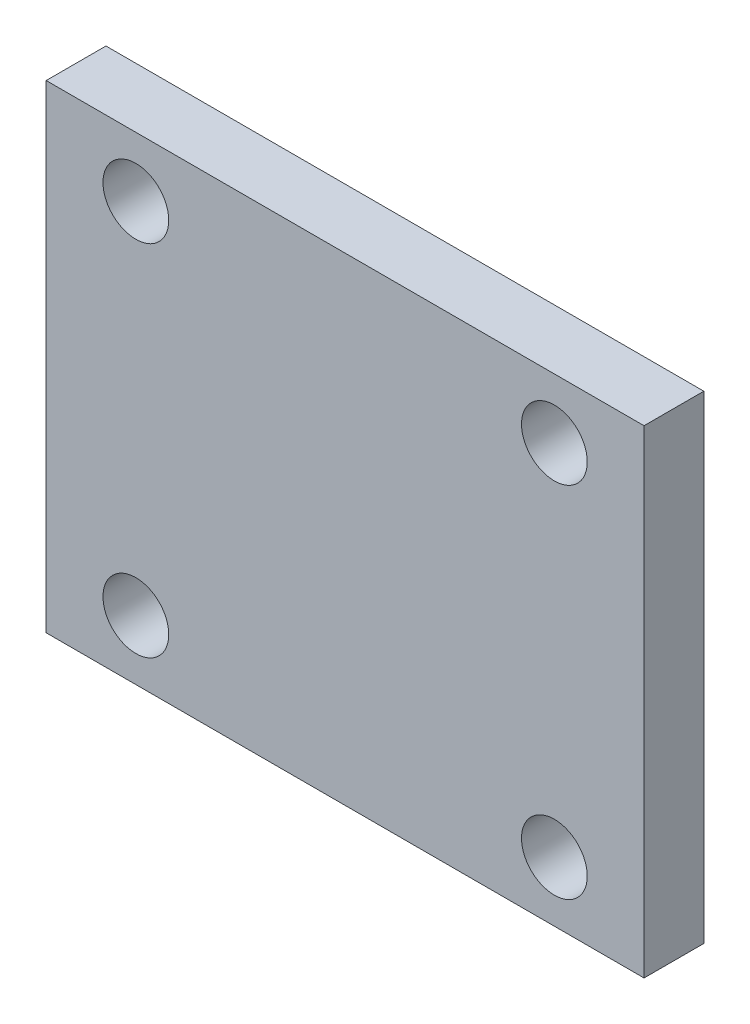
SolidWorks part; units mm, degrees
ref_plane "前视基准面" through (0, 0, 0) normal (0, 0, 1) x (1, 0, 0)
ref_plane "上视基准面" through (0, 0, 0) normal (0, 1, 0) x (1, 0, 0)
ref_plane "右视基准面" through (0, 0, 0) normal (1, 0, 0) x (0, 0, -1)
sketch "草图1" plane through (0, 0, 0) normal (0, 0, 1) x (1, 0, 0)
  line L1 (-50, -40) -> (50, -40)
  line L2 (-50, -40) -> (-50, 40)
  line L3 (-50, 40) -> (50, 40)
  line L4 (50, -40) -> (50, 40)
  line L5 (-50, -40) -> (50, 40) construction
  line L6 (-50, 40) -> (50, -40) construction
  circle A0 centre (-35, 30) radius 5.5
  circle A1 centre (-35, -30) radius 5.5
  circle A2 centre (35, -30) radius 5.5
  circle A3 centre (35, 30) radius 5.5
  point P0 (0, 0)
  dimension "D3" = 11
  dimension "D4" = 10
  dimension "D5" = 15
  dimension "D6" = 11
  dimension "D8" = 11
  dimension "D9" = 15
  dimension "D10" = 10
  dimension "D11" = 11
  dimension "D1" = 80
  dimension "D2" = 100
  dimension "D7" = 10
extrude "凸台-拉伸1" add sketch "草图1" along normal blind 10
